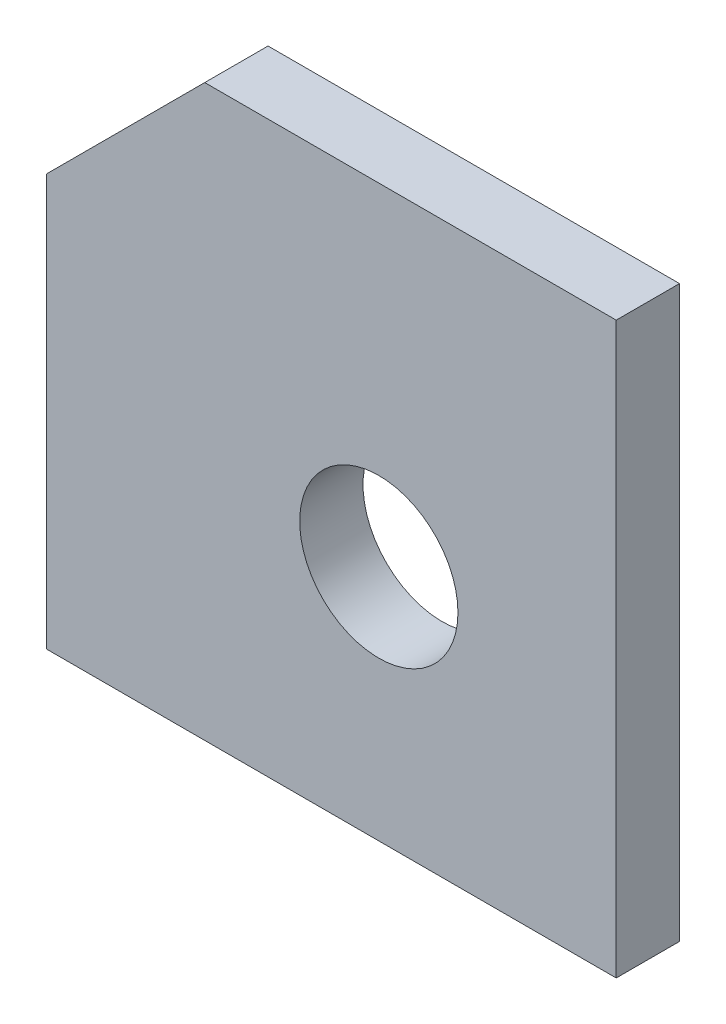
SolidWorks part; units mm, degrees
material "Q235"
ref_plane "前视基准面" through (0, 0, 0) normal (0, 0, 1) x (1, 0, 0)
ref_plane "上视基准面" through (0, 0, 0) normal (0, 1, 0) x (1, 0, 0)
ref_plane "右视基准面" through (0, 0, 0) normal (1, 0, 0) x (0, 0, -1)
sketch "草图1" plane through (0, 0, 0) normal (0, 0, 1) x (1, 0, 0)
  line L1 (0, 0) -> (36, 0)
  line L2 (0, 0) -> (0, 36)
  line L3 (0, 36) -> (36, 36)
  line L4 (36, 0) -> (36, 36)
  dimension "D1" = 36
  dimension "D2" = 36
extrude "凸台-拉伸1" add sketch "草图1" along normal blind 4
chamfer "倒角1" distance 10 angle 45 1 edges at (0, 36, 2)
hole_wizard "Ø10.0 (10) 直径孔1" positions "草图5" profile "草图4" hole size "Ø10.0" standard "Gb" end condition through all
sketch "草图5" plane through (0, 0, 4) normal (0, 0, 1) x (1, 0, 0)
  line L0 (36, 0) -> (36, 36) construction
  line L1 (0, 0) -> (36, 0) construction
  point P0 (21, 15)
  dimension "D1" = 15
  dimension "D2" = 15
sketch "草图4" plane through (21, 15, 4) normal (1, 0, 0) x (0, -1, 0)
  line L0 (0, 0) -> (0, 4)
  line L1 (0, 4) -> (5, 4)
  line L2 (5, 4) -> (5, 0)
  line L5 (5, 0) -> (0, 0)
  line L11 (0, -6.35) -> (0, 107.95) construction
  dimension "通孔孔直径" = 10
  dimension "通孔孔深度" = 4
